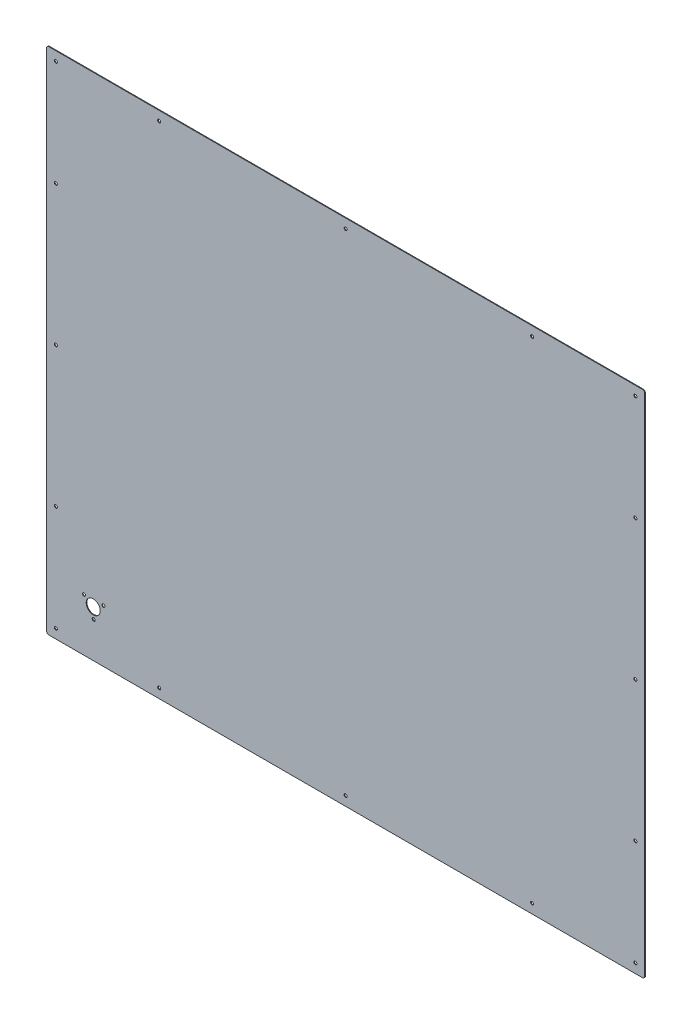
from build123d import *

# Parameters (mm, degrees)
SKETCH_1_W                  = 1283
SKETCH_1_H                  = 1093
EXTRUDE_1_DEPTH             = 1.5
FILLET_1_R                  = 5
HOLE_WIZARD_6_5_6_5_1_D     = 6.5
HOLE_WIZARD_6_5_6_5_1_DEPTH = 15.61
HOLE_WIZARD_6_5_6_5_1_TIP   = 1.876388375
SKETCH_5_R                  = 15
CUT_EXTRUDE_1_DEPTH         = 10
HOLE_WIZARD_6_5_6_5_2_D     = 6.5
HOLE_WIZARD_6_5_6_5_2_DEPTH = 15.61
HOLE_WIZARD_6_5_6_5_2_TIP   = 1.876388375


with BuildPart() as part:
    # 草图1 → 凸台-拉伸1 (new body)
    with BuildSketch(Plane.XY):
        Rectangle(SKETCH_1_W, SKETCH_1_H)
    extrude(amount=EXTRUDE_1_DEPTH)

    # 圆角1
    fillet_1_edges = [part.edges().sort_by_distance(p)[0] for p in [
        (-641.5, 546.5, 0.75),
        (641.5, 546.5, 0.75),
        (641.5, -546.5, 0.75),
        (-641.5, -546.5, 0.75),
    ]]
    fillet(fillet_1_edges, radius=FILLET_1_R)

    # Ø6.5 (6.5) 直径孔1
    with Locations(Plane.XY.offset(1.5)):
        with Locations((0, 526.5), (400, 526.5), (-400, 526.5), (-621.5, 300), (-621.5, 0), (-621.5, -300), (-400, -526.5), (0, -526.5), (400, -526.5), (621.5, 300), (621.5, 0), (621.5, -300), (-621.5, 526.5), (-621.5, -526.5), (621.5, -526.5), (621.5, 526.5)):
            Hole(HOLE_WIZARD_6_5_6_5_1_D / 2, depth=HOLE_WIZARD_6_5_6_5_1_DEPTH)
            with Locations((0, 0, -(HOLE_WIZARD_6_5_6_5_1_DEPTH + HOLE_WIZARD_6_5_6_5_1_TIP / 2))):  # 120° drill point
                Cone(0, HOLE_WIZARD_6_5_6_5_1_D / 2, HOLE_WIZARD_6_5_6_5_1_TIP, mode=Mode.SUBTRACT)

    # 草图5 → 切除-拉伸1 (cut)
    with BuildSketch(Plane.XY.offset(1.5)):
        with Locations((-541.5, -446.5)):
            Circle(SKETCH_5_R)
    extrude(amount=-CUT_EXTRUDE_1_DEPTH, mode=Mode.SUBTRACT)

    # Ø6.5 (6.5) 直径孔2
    with Locations(Plane.XY.offset(1.5)):
        with Locations((-561.284609691, -433.5), (-540.5, -469.5), (-519.715390309, -433.5)):
            Hole(HOLE_WIZARD_6_5_6_5_2_D / 2, depth=HOLE_WIZARD_6_5_6_5_2_DEPTH)
            with Locations((0, 0, -(HOLE_WIZARD_6_5_6_5_2_DEPTH + HOLE_WIZARD_6_5_6_5_2_TIP / 2))):  # 120° drill point
                Cone(0, HOLE_WIZARD_6_5_6_5_2_D / 2, HOLE_WIZARD_6_5_6_5_2_TIP, mode=Mode.SUBTRACT)


solid = part.part
